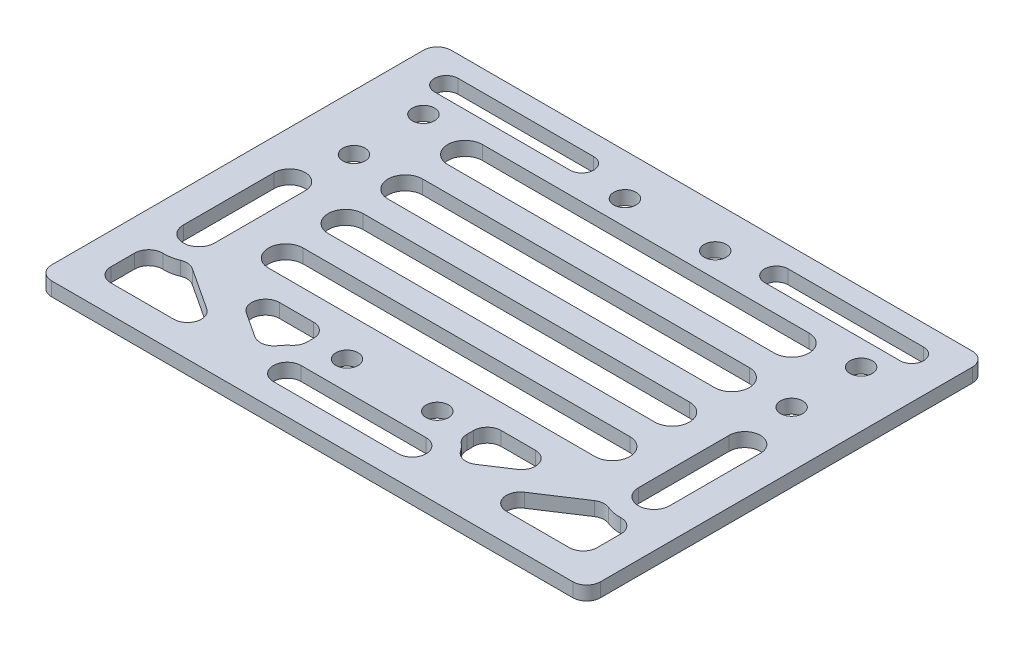
SolidWorks part; units mm, degrees
material "Thornel Mat VMA"
ref_plane "前视基准面" through (0, 0, 0) normal (0, 0, 1) x (1, 0, 0)
ref_plane "上视基准面" through (0, 0, 0) normal (0, 1, 0) x (1, 0, 0)
ref_plane "右视基准面" through (0, 0, 0) normal (1, 0, 0) x (0, 0, -1)
sketch "草图1" plane through (0, 0, 0) normal (0, 1, 0) x (1, 0, 0)
  line L0 (-31.5, 18.75) -> (-31.5, 8.75) construction
  line L1 (-39.5, 28.75) -> (39.5, 28.75)
  line L2 (-39.5, 28.75) -> (-39.5, -28.75)
  line L3 (-39.5, -28.75) -> (39.5, -28.75)
  line L4 (39.5, 28.75) -> (39.5, -28.75)
  line L5 (-39.5, 28.75) -> (39.5, -28.75) construction
  line L6 (-39.5, -28.75) -> (39.5, 28.75) construction
  line L7 (0, 28.75) -> (0, -28.75) construction
  line L8 (31.5, 18.75) -> (31.5, 8.75) construction
  line L9 (-6.5, 22.75) -> (6.5, 22.75) construction
  line L10 (-6.5, -17.25) -> (6.5, -17.25) construction
  circle A0 centre (-31.5, 18.75) radius 1.6
  circle A1 centre (-31.5, 8.75) radius 1.6
  circle A2 centre (31.5, 8.75) radius 1.6
  circle A3 centre (31.5, 18.75) radius 1.6
  circle A4 centre (-6.5, 22.75) radius 1.6
  circle A5 centre (-6.5, -17.25) radius 1.6
  circle A6 centre (6.5, 22.75) radius 1.6
  circle A7 centre (6.5, -17.25) radius 1.6
  point P0 (0, 0)
  dimension "D3" = 3.2
  dimension "D7" = 13
  dimension "D1" = 79
  dimension "D2" = 57.5
  dimension "D4" = 8
  dimension "D5" = 37.5
  dimension "D6" = 10
  dimension "D8" = 11.5
  dimension "D9" = 6
extrude "凸台-拉伸1" add sketch "草图1" along normal blind 2
sketch "草图2" plane through (0, 2, 0) normal (0, 1, 0) x (1, 0, 0)
  line L0 (0, 28.75) -> (0, -28.75) construction
  line L1 (39.5, 28.75) -> (-39.5, 28.75) construction
  line L2 (-39.5, -28.75) -> (39.5, -28.75) construction
  line L3 (-23.5, 16.75) -> (23.5, 16.75) construction
  line L4 (-23.5, 19.25) -> (23.5, 19.25)
  line L5 (-23.5, 14.25) -> (23.5, 14.25)
  line L6 (-6.5, 22.75) -> (6.5, 22.75) construction
  line L7 (-6.5, -17.25) -> (6.5, -17.25) construction
  line L8 (-31.5, 18.75) -> (-31.5, 8.75) construction
  line L9 (31.5, 18.75) -> (31.5, 8.75) construction
  line L10 (-23.5, 8.15) -> (23.5, 8.15) construction
  line L11 (-23.5, 10.65) -> (23.5, 10.65)
  line L12 (-23.5, 5.65) -> (23.5, 5.65)
  line L13 (-23.5, -0.45) -> (23.5, -0.45) construction
  line L14 (-23.5, 2.05) -> (23.5, 2.05)
  line L15 (-23.5, -2.95) -> (23.5, -2.95)
  line L16 (-23.5, -9.05) -> (23.5, -9.05) construction
  line L19 (-23.5, -6.55) -> (23.5, -6.55)
  line L24 (-39.5, 28.75) -> (-39.5, -28.75) construction
  line L25 (-33.5, 24.05) -> (-14, 24.05) construction
  line L26 (-33.5, 25.75) -> (-14, 25.75)
  line L27 (-33.5, 22.35) -> (-14, 22.35)
  line L28 (33.5, 24.05) -> (14, 24.05) construction
  line L29 (33.5, 25.75) -> (14, 25.75)
  line L30 (33.5, 22.35) -> (14, 22.35)
  line L31 (-23.5, -11.55) -> (23.5, -11.55)
  line L32 (-9, -23.35) -> (9, -23.35) construction
  line L33 (-9, -21.35) -> (9, -21.35)
  line L34 (-9, -25.35) -> (9, -25.35)
  line L35 (-32.75, 0.75) -> (-32.75, -12.3054) construction
  line L36 (-30.5, 0.75) -> (-30.5, -12.3054)
  line L37 (-35, 0.75) -> (-35, -12.3054)
  line L38 (32.75, 0.75) -> (32.75, -12.3054) construction
  line L39 (30.5, 0.75) -> (30.5, -12.3054)
  line L40 (35, 0.75) -> (35, -12.3054)
  line L41 (-35, -16.7705) -> (-35, -24.75)
  line L42 (-35, -24.75) -> (-17.2613, -24.75)
  line L43 (-25.1093, -15.05) -> (-11.5, -15.05)
  line L44 (-11.5, -15.05) -> (-11.5, -19.0199)
  line L45 (-28.5706, -15.05) -> (-13.8, -24.75) construction
  line L46 (-17.2613, -24.75) -> (-29.9271, -16.4323)
  line L47 (-13.9098, -22.4048) -> (-25.1093, -15.05)
  line L48 (17.2613, -24.75) -> (29.9271, -16.4323)
  line L49 (35, -24.75) -> (17.2613, -24.75)
  line L50 (35, -16.7705) -> (35, -24.75)
  line L51 (25.1093, -15.05) -> (11.5, -15.05)
  line L52 (13.9098, -22.4048) -> (25.1093, -15.05)
  line L53 (11.5, -15.05) -> (11.5, -19.0199)
  arc A0 (-23.5, 19.25) -> (-23.5, 14.25) centre (-23.5, 16.75) ccw
  arc A1 (23.5, 14.25) -> (23.5, 19.25) centre (23.5, 16.75) ccw
  arc A2 (-23.5, 10.65) -> (-23.5, 5.65) centre (-23.5, 8.15) ccw
  arc A3 (23.5, 5.65) -> (23.5, 10.65) centre (23.5, 8.15) ccw
  arc A4 (-23.5, 2.05) -> (-23.5, -2.95) centre (-23.5, -0.45) ccw
  arc A5 (23.5, -2.95) -> (23.5, 2.05) centre (23.5, -0.45) ccw
  arc A12 (-33.5, 25.75) -> (-33.5, 22.35) centre (-33.5, 24.05) ccw
  arc A13 (-14, 22.35) -> (-14, 25.75) centre (-14, 24.05) ccw
  arc A14 (33.5, 25.75) -> (33.5, 22.35) centre (33.5, 24.05) cw
  arc A15 (14, 22.35) -> (14, 25.75) centre (14, 24.05) cw
  arc A16 (-23.5, -6.55) -> (-23.5, -11.55) centre (-23.5, -9.05) ccw
  arc A17 (23.5, -11.55) -> (23.5, -6.55) centre (23.5, -9.05) ccw
  arc A18 (-9, -21.35) -> (-9, -25.35) centre (-9, -23.35) ccw
  arc A19 (9, -25.35) -> (9, -21.35) centre (9, -23.35) ccw
  arc A20 (-30.5, 0.75) -> (-35, 0.75) centre (-32.75, 0.75) ccw
  arc A21 (-35, -12.3054) -> (-30.5, -12.3054) centre (-32.75, -12.3054) ccw
  arc A22 (30.5, 0.75) -> (35, 0.75) centre (32.75, 0.75) cw
  arc A23 (35, -12.3054) -> (30.5, -12.3054) centre (32.75, -12.3054) cw
  arc A24 (-35, -16.7705) -> (-29.9271, -16.4323) centre (-32.75, -12.3054) ccw
  arc A25 (-11.5, -19.0199) -> (-13.9098, -22.4048) centre (-9, -23.35) ccw
  arc A26 (35, -16.7705) -> (29.9271, -16.4323) centre (32.75, -12.3054) cw
  arc A27 (11.5, -19.0199) -> (13.9098, -22.4048) centre (9, -23.35) cw
  point P8 (0, 16.75)
  point P32 (0, 8.15)
  point P39 (0, -0.45)
  point P45 (0, -9.05)
  point P52 (0, -23.35)
  point P61 (-23.75, 24.05)
  point P68 (23.75, 24.05)
  point P75 (-32.75, -5.7777)
  point P82 (32.75, -5.7777)
  point P91 (0, 0)
  point P99 (-32.75, -12.9097)
  point P101 (0, 0)
  dimension "D2" = 2.5
  dimension "D15" = 4
  dimension "D16" = 5
  dimension "D17" = 5
  dimension "D1" = 3.5
  dimension "D3" = 8
  dimension "D5" = 4
  dimension "D6" = 3.4
  dimension "D7" = 3.6
  dimension "D8" = 4.5
  dimension "D9" = 3
  dimension "D10" = 28
  dimension "D11" = 3.4
  dimension "D12" = 6
  dimension "D13" = 4.5
  dimension "D14" = 8
  dimension "D18" = 18
  dimension "D19" = 3.5
  dimension "D20" = 5
  dimension "D21" = 3.8
  dimension "D4" = 4
extrude "切除-拉伸1" cut sketch "草图2" against normal through all
fillet "R2 圆角1" radius 2 20 edges at (39.5, 1, 28.75) (-39.5, 1, -28.75) (39.5, 1, -28.75) (-39.5, 1, 28.75) (35, 1, 24.75) (17.2613, 1, 24.75) (29.9271, 1, 16.4323) (35, 1, 16.7705) (11.5, 1, 19.0199) (11.5, 1, 15.05) (25.1093, 1, 15.05) (13.9098, 1, 22.4048) (-17.2613, 1, 24.75) (-35, 1, 24.75) (-29.9271, 1, 16.4323) (-13.9098, 1, 22.4048) (-25.1093, 1, 15.05) (-11.5, 1, 15.05) (-11.5, 1, 19.0199) (-35, 1, 16.7705)
